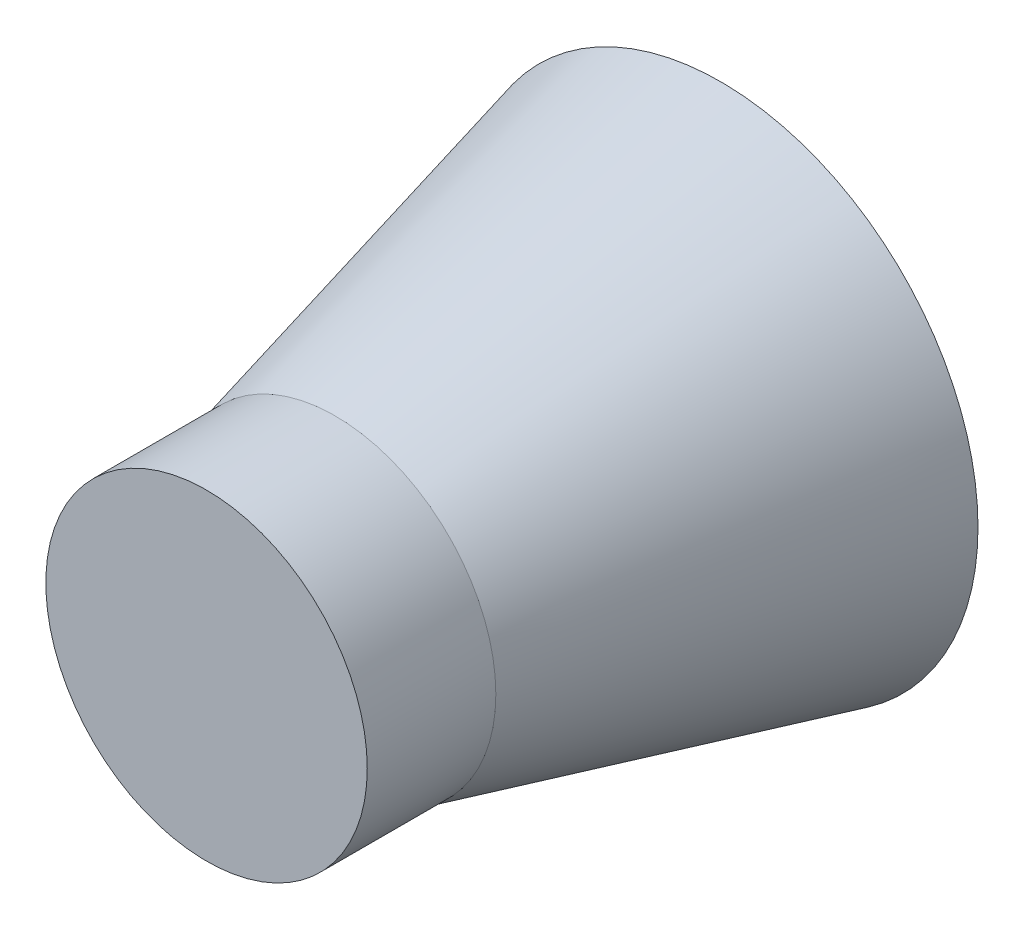
SolidWorks part; units mm, degrees
ref_plane "Front Plane" through (0, 0, 0) normal (0, 0, 1) x (1, 0, 0)
ref_plane "Top Plane" through (0, 0, 0) normal (0, 1, 0) x (1, 0, 0)
ref_plane "Right Plane" through (0, 0, 0) normal (1, 0, 0) x (0, 0, -1)
other "Configuration Table"
sketch "Sketch1" plane through (0, 0, 0) normal (0, 0, 1) x (1, 0, 0)
  circle A0 centre (0, 0) radius 20
  dimension "D1" = 40
ref_plane "Plane1" through (0, 0, 30) normal (0, 0, -1) x (-1, 0, 0)
sketch "Sketch2" plane through (0, 0, 30) normal (0, 0, -1) x (-1, 0, 0)
  circle A0 centre (0, 0) radius 12.5
  dimension "D1" = 25
loft "Loft1" add profiles "Sketch2", "Sketch1"
sketch "Sketch3" plane through (0, 0, 30) normal (0, 0, 1) x (1, 0, 0)
  circle A0 centre (0, 0) radius 12.5
extrude "Boss-Extrude1" add sketch "Sketch3" along normal blind 10
